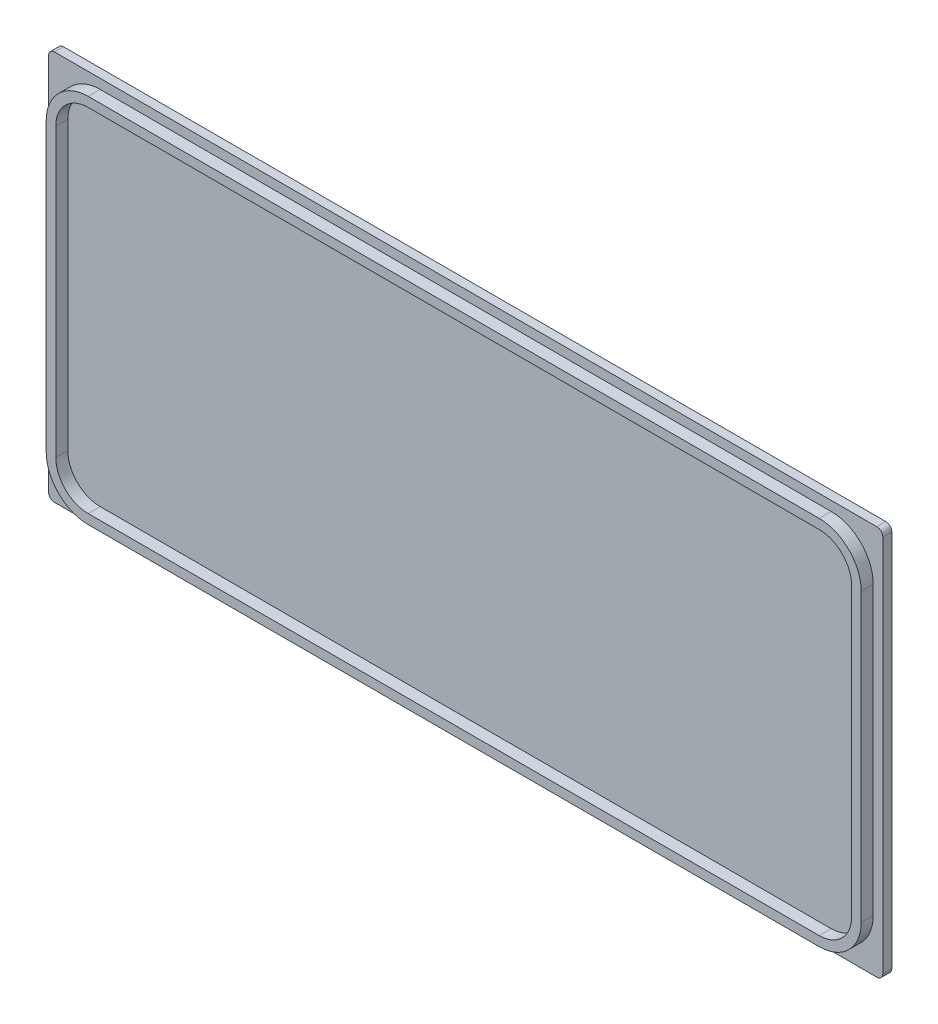
SolidWorks part; units mm, degrees
ref_plane "Front Plane" through (0, 0, 0) normal (0, 0, 1) x (1, 0, 0)
ref_plane "Top Plane" through (0, 0, 0) normal (0, 1, 0) x (1, 0, 0)
ref_plane "Right Plane" through (0, 0, 0) normal (1, 0, 0) x (0, 0, -1)
other "Configuration Table"
sketch "Sketch1" plane through (0, 0, 0) normal (0, 0, 1) x (1, 0, 0)
  line L1 (-68.5, 32.5) -> (68.5, 32.5)
  line L2 (-69.5, 31.5) -> (-69.5, -31.5)
  line L3 (-68.5, -32.5) -> (68.5, -32.5)
  line L4 (69.5, 31.5) -> (69.5, -31.5)
  line L5 (-69.5, 32.5) -> (69.5, -32.5) construction
  line L6 (-69.5, -32.5) -> (69.5, 32.5) construction
  arc A0 (-69.5, -31.5) -> (-68.5, -32.5) centre (-68.5, -31.5) ccw
  arc A1 (68.5, -32.5) -> (69.5, -31.5) centre (68.5, -31.5) ccw
  arc A2 (68.5, 32.5) -> (69.5, 31.5) centre (68.5, 31.5) cw
  arc A3 (-68.5, 32.5) -> (-69.5, 31.5) centre (-68.5, 31.5) ccw
  point P0 (0, 0)
  dimension "D3" = 1
  dimension "D1" = 139
  dimension "D2" = 65
extrude "Boss-Extrude1" add sketch "Sketch1" along normal blind 1.5
sketch "Sketch2" plane through (0, 0, 1.5) normal (0, 0, 1) x (1, 0, 0)
  line L1 (-58, 18) -> (58, 18) construction
  line L2 (-58, 18) -> (-58, -18) construction
  line L3 (-58, -18) -> (58, -18) construction
  line L4 (58, 18) -> (58, -18) construction
  line L5 (-58, 18) -> (58, -18) construction
  line L6 (-58, -18) -> (58, 18) construction
  circle A0 centre (-58, 18) radius 6
  circle A1 centre (-58, 18) radius 5.1
  circle A2 centre (58, 18) radius 6
  circle A3 centre (58, 18) radius 5.1
  circle A4 centre (-58, -18) radius 6
  circle A5 centre (-58, -18) radius 5.1
  circle A6 centre (58, -18) radius 6
  circle A7 centre (58, -18) radius 5.1
  point P0 (0, 0)
  dimension "D1" = 12
  dimension "D2" = 10.2
  dimension "D3" = 116
  dimension "D4" = 36
extrude "Boss-Extrude2" add sketch "Sketch2" against normal blind 1 from offset 1.5 offset against normal yes
sketch "Sketch3" plane through (0, 0, 1.5) normal (0, 0, 1) x (1, 0, 0)
  line L0 (60.9, 30.9) -> (-60.9, 30.9)
  line L1 (-67.9, 23.9) -> (-67.9, -23.9)
  line L2 (-60.9, -30.9) -> (60.9, -30.9)
  line L3 (67.9, -23.9) -> (67.9, 23.9)
  line L16 (68.5, 32.5) -> (-68.5, 32.5) construction
  line L17 (-68.5, -32.5) -> (68.5, -32.5) construction
  line L18 (60.9, 29.3) -> (-60.9, 29.3)
  line L19 (69.5, -31.5) -> (69.5, 31.5) construction
  line L20 (-66.3, 23.9) -> (-66.3, -23.9)
  line L21 (-69.5, 31.5) -> (-69.5, -31.5) construction
  line L22 (-60.9, -29.3) -> (60.9, -29.3)
  line L23 (66.3, -23.9) -> (66.3, 23.9)
  arc A16 (-60.9, 30.9) -> (-67.9, 23.9) centre (-60.9, 23.9) ccw
  arc A17 (60.9, -30.9) -> (67.9, -23.9) centre (60.9, -23.9) ccw
  arc A18 (67.9, 23.9) -> (60.9, 30.9) centre (60.9, 23.9) ccw
  arc A19 (-67.9, -23.9) -> (-60.9, -30.9) centre (-60.9, -23.9) ccw
  arc A20 (-60.9, 29.3) -> (-66.3, 23.9) centre (-60.9, 23.9) ccw
  arc A21 (-66.3, -23.9) -> (-60.9, -29.3) centre (-60.9, -23.9) ccw
  arc A22 (60.9, -29.3) -> (66.3, -23.9) centre (60.9, -23.9) ccw
  arc A23 (66.3, 23.9) -> (60.9, 29.3) centre (60.9, 23.9) ccw
  dimension "D1" = 7
  dimension "D2" = 1.6
  dimension "D3" = 1.6
  dimension "D4" = 1.6
  dimension "D5" = 1.6
  dimension "D6" = 1.6
extrude "Boss-Extrude3" add sketch "Sketch3" along normal blind 2
sketch "Sketch7" plane through (0, -32.5, 0) normal (0, -1, 0) x (-1, 0, 0)
  line L1 (1, -9.7058) -> (-1, -9.7058)
  line L2 (1, -9.7058) -> (1, 9.7058)
  line L3 (1, 9.7058) -> (-1, 9.7058)
  line L4 (-1, -9.7058) -> (-1, 9.7058)
  line L5 (1, -9.7058) -> (-1, 9.7058) construction
  line L6 (1, 9.7058) -> (-1, -9.7058) construction
  point P0 (0, 0)
  dimension "D1" = 2
extrude "Cut-Extrude3" cut sketch "Sketch7" against normal blind 0.8
sketch "Sketch8" plane through (0, 0, 0) normal (0, 0, -1) x (-1, 0, 0)
  circle A0 centre (-58, 18) radius 5.1
  circle A1 centre (58, 18) radius 5.1
  circle A2 centre (58, -18) radius 5.1
  circle A3 centre (-58, -18) radius 5.1
extrude "Cut-Extrude4" cut sketch "Sketch8" against normal blind 1
